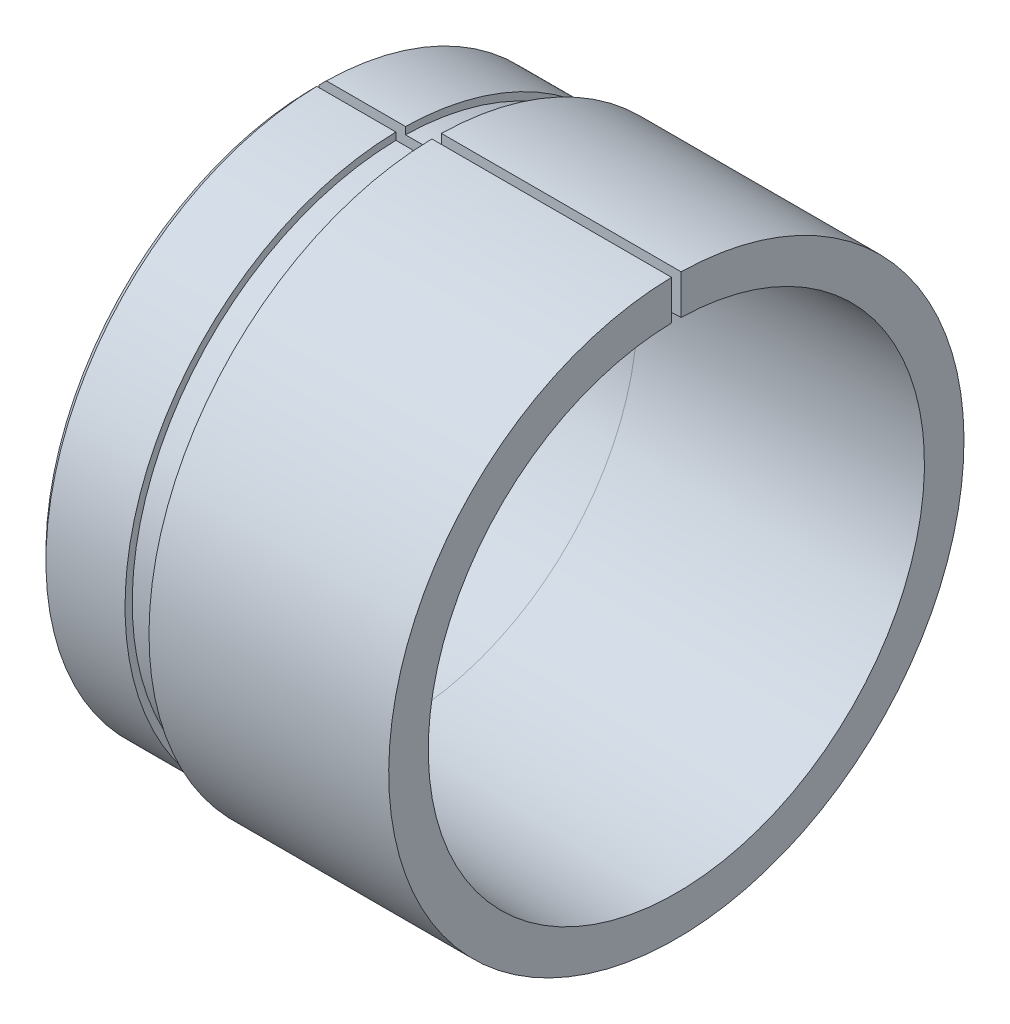
SolidWorks part; units mm, degrees
material "45"
ref_plane "Front Plane" through (0, 0, 0) normal (0, 0, 1) x (1, 0, 0)
ref_plane "Top Plane" through (0, 0, 0) normal (0, 1, 0) x (1, 0, 0)
ref_plane "Right Plane" through (0, 0, 0) normal (1, 0, 0) x (0, 0, -1)
sketch "Sketch1" plane through (0, 0, 0) normal (0, 0, 1) x (1, 0, 0)
  line L0 (0, 0) -> (200.2579, 0) construction
  line L1 (0, 115) -> (36, 115)
  line L2 (36, 115) -> (36, 112)
  line L3 (36, 112) -> (51, 112)
  line L4 (51, 112) -> (51, 120)
  line L5 (51, 120) -> (151, 120)
  line L6 (151, 120) -> (151, 103.5)
  line L7 (151, 103.5) -> (36, 98.7)
  line L8 (36, 98.7) -> (0, 98.7)
  line L9 (0, 98.7) -> (0, 115)
  dimension "D1" = 98.7
  dimension "D2" = 115
  dimension "D3" = 112
  dimension "D4" = 120
  dimension "D5" = 103.5
  dimension "D6" = 151
  dimension "D7" = 100
  dimension "D8" = 15
revolve "Revolve1" add sketch "Sketch1" angle 360 about L0
chamfer "Chamfer1" distance 3 angle 45 1 edges at (0, 0, 115)
sketch "Sketch2" plane through (0, 0, 0) normal (1, 0, 0) x (0, 0, -1)
  line L0 (0, 0) -> (0, 153.1069) construction
  line L2 (2, 68.3094) -> (-2, 68.3094)
  line L3 (2, 68.3094) -> (2, 138.6906)
  line L4 (2, 138.6906) -> (-2, 138.6906)
  line L5 (-2, 68.3094) -> (-2, 138.6906)
  line L6 (2, 68.3094) -> (-2, 138.6906) construction
  line L7 (2, 138.6906) -> (-2, 68.3094) construction
  circle A0 centre (0, 0) radius 103.5 construction
  point P3 (0, 103.5)
  dimension "D1" = 4
extrude "Cut-Extrude2" cut sketch "Sketch2" along normal through all
